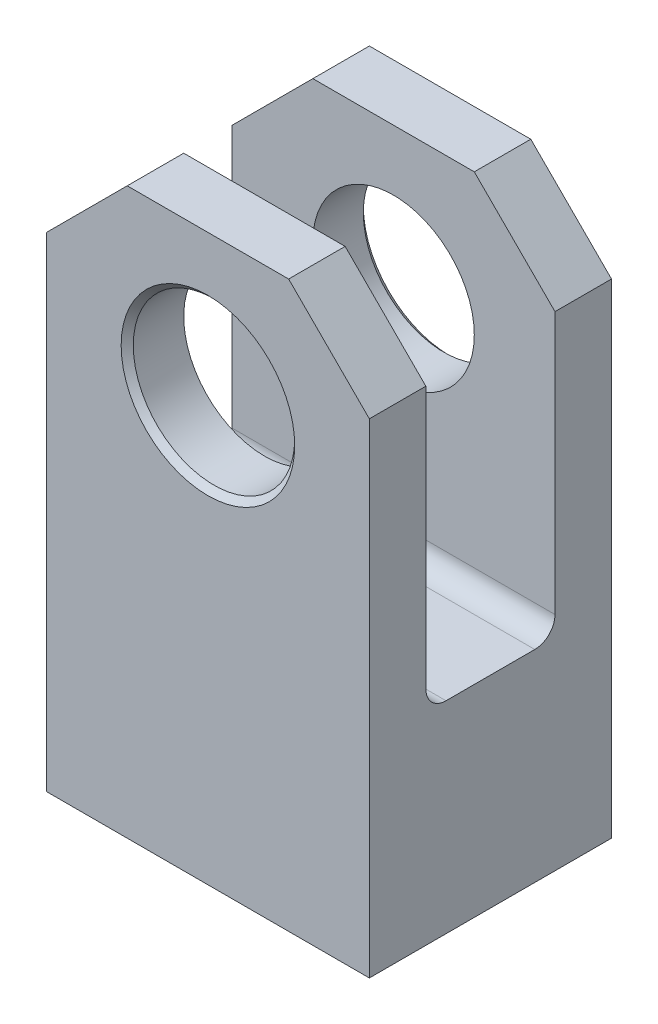
from build123d import *

# Parameters (mm, degrees)
SKETCH2_W               = 80
SKETCH2_H               = 140
BOSS_EXTRUDE1_DEPTH     = 30
CHAMFER1_SIZE           = 20
CUT_EXTRUDE1_DEPTH      = 111.453610172
CUT_EXTRUDE1_DEPTH_BACK = 111.453610172
SKETCH3_W               = 32
SKETCH3_H               = 180
FILLET1_R               = 5
CUT_EXTRUDE2_DEPTH      = 101.498756211
CUT_EXTRUDE2_DEPTH_BACK = 101.498756211
SKETCH4_R               = 20
CHAMFER2_SIZE           = 1.5
M24_TAPPED_HOLE1_D      = 21


with BuildPart() as part:
    # Sketch2 → Boss-Extrude1 (new, symmetric)
    with BuildSketch(Plane.XY):
        Rectangle(SKETCH2_W, SKETCH2_H)
    extrude(amount=BOSS_EXTRUDE1_DEPTH, both=True)

    # Chamfer1
    chamfer1_edges = [part.edges().sort_by_distance(p)[0] for p in [
        (-40, 70, 0),
        (40, 70, 0),
    ]]
    chamfer(chamfer1_edges, length=CHAMFER1_SIZE)

    # Sketch3 → Cut-Extrude1 (cut, two sides: drawn at the far end of the back side and taken through both)
    with BuildSketch(Plane.ZY.offset(40).offset(-CUT_EXTRUDE1_DEPTH_BACK)):
        with Locations((0, 70)):
            Rectangle(SKETCH3_W, SKETCH3_H)
    extrude(amount=CUT_EXTRUDE1_DEPTH + CUT_EXTRUDE1_DEPTH_BACK, mode=Mode.SUBTRACT)

    # Fillet1
    fillet1_edges = [part.edges().sort_by_distance(p)[0] for p in [
        (0, -20, 16),
        (0, -20, -16),
    ]]
    fillet(fillet1_edges, radius=FILLET1_R)

    # Sketch4 → Cut-Extrude2 (cut, two sides: drawn at the far end of the back side and taken through both)
    with BuildSketch(Plane.XY.offset(30).offset(-CUT_EXTRUDE2_DEPTH_BACK)):
        with Locations((0, 35)):
            Circle(SKETCH4_R)
    extrude(amount=CUT_EXTRUDE2_DEPTH + CUT_EXTRUDE2_DEPTH_BACK, mode=Mode.SUBTRACT)

    # Chamfer2
    chamfer2_edges = [part.edges().sort_by_distance(p)[0] for p in [
        (-20, 35, 30),
        (-20, 35, -30),
    ]]
    chamfer(chamfer2_edges, length=CHAMFER2_SIZE)

    # M24 Tapped Hole1 (through all)
    with Locations(Plane(origin=(0, -20, 0), x_dir=(1, 0, 0), z_dir=(0, 1, 0))):
        with Locations((0, 0)):
            Hole(M24_TAPPED_HOLE1_D / 2)


solid = part.part
